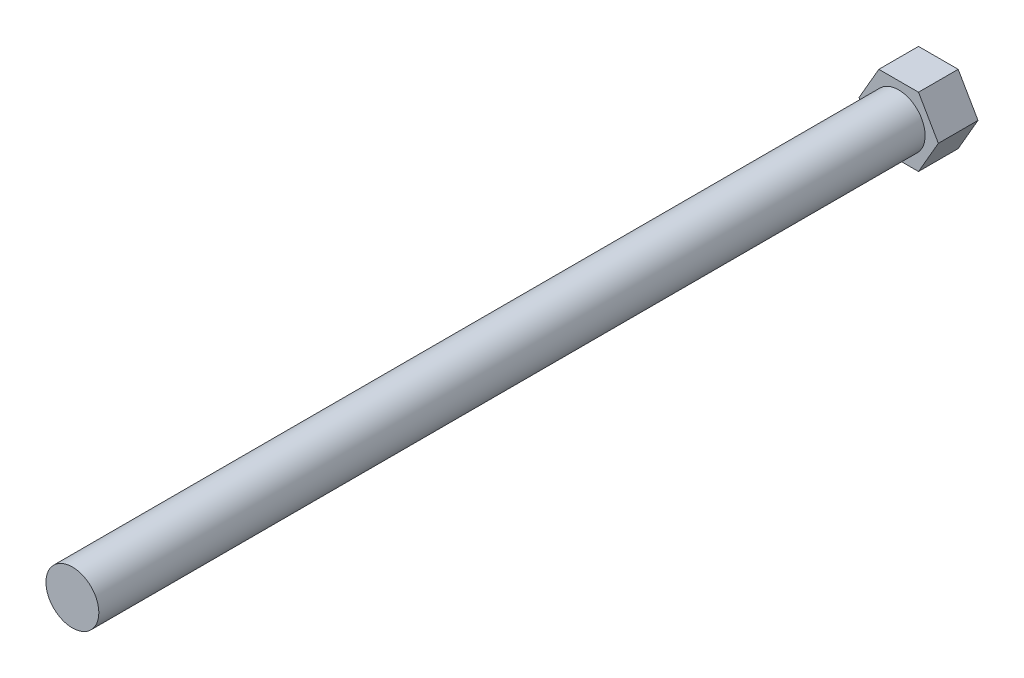
SolidWorks part; units mm, degrees
ref_plane "前视基准面" through (0, 0, 0) normal (0, 0, 1) x (1, 0, 0)
ref_plane "上视基准面" through (0, 0, 0) normal (0, 1, 0) x (1, 0, 0)
ref_plane "右视基准面" through (0, 0, 0) normal (1, 0, 0) x (0, 0, -1)
other "Configuration Table"
sketch "草图1" plane through (0, 0, 0) normal (0, 0, 1) x (1, 0, 0)
  circle A0 centre (0, 0) radius 8
  point P0 (0, 0)
  dimension "D1" = 16
extrude "凸台-拉伸1" add sketch "草图1" along normal blind 250
sketch "草图2" plane through (0, 0, 0) normal (0, 0, 1) x (1, 0, 0)
  line L0 (12, 0) -> (6, 10.3923)
  line L1 (6, 10.3923) -> (-6, 10.3923)
  line L2 (-6, 10.3923) -> (-12, 0)
  line L3 (-12, 0) -> (-6, -10.3923)
  line L4 (-6, -10.3923) -> (6, -10.3923)
  line L5 (6, -10.3923) -> (12, 0)
  point P0 (0, 0)
  dimension "D1" = 6
  dimension "D2" = 12
  dimension "D3" = 18
  dimension "D4" = 24
  dimension "D5" = 10.3923
  dimension "D6" = 20.7846
extrude "凸台-拉伸2" add sketch "草图2" against normal blind 12
